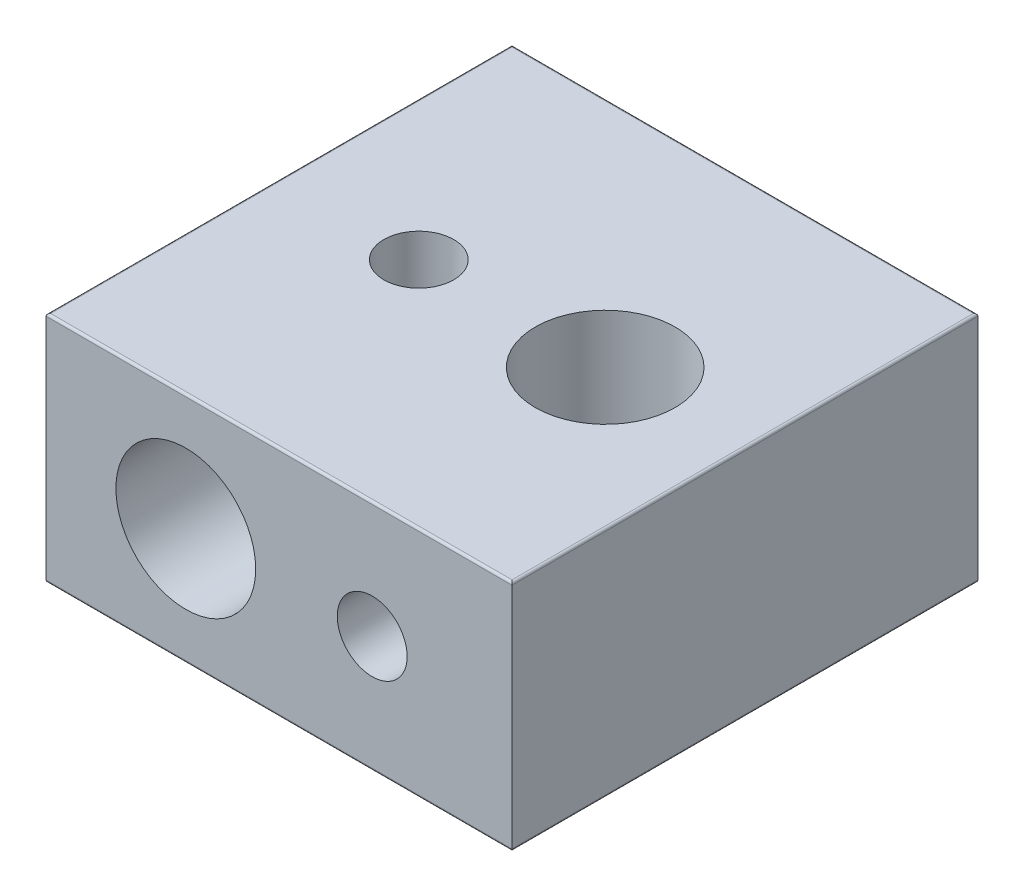
from build123d import *

# Parameters (mm, degrees)
SKETCH1_W           = 20
SKETCH1_H           = 20
SKETCH1_R           = 1.5
SKETCH1_R_2         = 3
BOSS_EXTRUDE1_DEPTH = 10
CUT_EXTRUDE5_START  = 10
SKETCH1_3_R         = 1.5
CUT_EXTRUDE5_DEPTH  = 5
SKETCH2_R           = 3
CUT_EXTRUDE1_DEPTH  = 31
SKETCH3_R           = 1.5
CUT_EXTRUDE2_DEPTH  = 3.5
FILLET1_R           = 0.1


with BuildPart() as part:
    # Sketch1 → Boss-Extrude1 (new body)
    # profile 1 of 2: a face of its own
    with BuildSketch(Plane(origin=(0, 0, 0), x_dir=(1, 0, 0), z_dir=(0, 1, 0))):
        with Locations((10, 10)):
            Rectangle(SKETCH1_W, SKETCH1_H)
        with Locations((6, 10)):
            Circle(SKETCH1_R, mode=Mode.SUBTRACT)
        with Locations(Location((14, 10, 0), (0, 0, 270))):
            Circle(SKETCH1_R_2, mode=Mode.SUBTRACT)
    # profile 2 of 2: a face of its own
    with BuildSketch(Plane(origin=(0, 0, 0), x_dir=(1, 0, 0), z_dir=(0, 1, 0))):
        with Locations((6, 10)):
            Circle(SKETCH1_R)
    extrude(amount=BOSS_EXTRUDE1_DEPTH)

    # Sketch1<3> → Cut-Extrude5 (cut)
    with BuildSketch(Plane(origin=(0, 0, 0), x_dir=(1, 0, 0), z_dir=(0, 1, 0)).offset(CUT_EXTRUDE5_START)):
        with Locations(Location((6, 10, 0), (0, 0, 270))):
            Circle(SKETCH1_3_R)
    extrude(amount=-CUT_EXTRUDE5_DEPTH, mode=Mode.SUBTRACT)

    # Sketch2 → Cut-Extrude1 (cut, through all)
    with BuildSketch(Plane.XY):
        with Locations((6, 5)):
            Circle(SKETCH2_R)
    extrude(amount=-CUT_EXTRUDE1_DEPTH, mode=Mode.SUBTRACT)

    # Sketch3 → Cut-Extrude2 (cut)
    with BuildSketch(Plane.XY):
        with Locations((14, 5)):
            Circle(SKETCH3_R)
    extrude(amount=-CUT_EXTRUDE2_DEPTH, mode=Mode.SUBTRACT)

    # Fillet1
    fillet1_edges = [part.edges().sort_by_distance(p)[0] for p in [
        (20, 10, -10),
        (10, 10, -20),
        (0, 10, -10),
        (0, 0, -10),
        (10, 0, -20),
        (20, 0, -10),
        (10, 0, 0),
        (10, 10, 0),
    ]]
    fillet(fillet1_edges, radius=FILLET1_R)


solid = part.part
